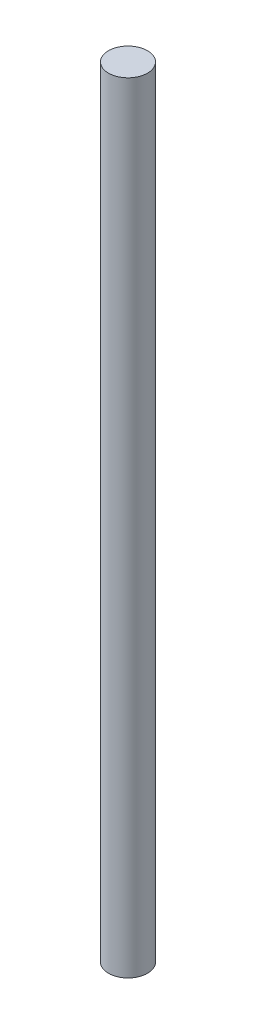
SolidWorks part; units mm, degrees
ref_plane "Front Plane" through (0, 0, 0) normal (0, 0, 1) x (1, 0, 0)
ref_plane "Top Plane" through (0, 0, 0) normal (0, 1, 0) x (1, 0, 0)
ref_plane "Right Plane" through (0, 0, 0) normal (1, 0, 0) x (0, 0, -1)
sketch "Sketch1" plane through (0, 0, 0) normal (0, 1, 0) x (1, 0, 0)
  circle A0 centre (0, 0) radius 10
  dimension "D1" = 20
extrude "Boss-Extrude1" add sketch "Sketch1" along normal blind 400
